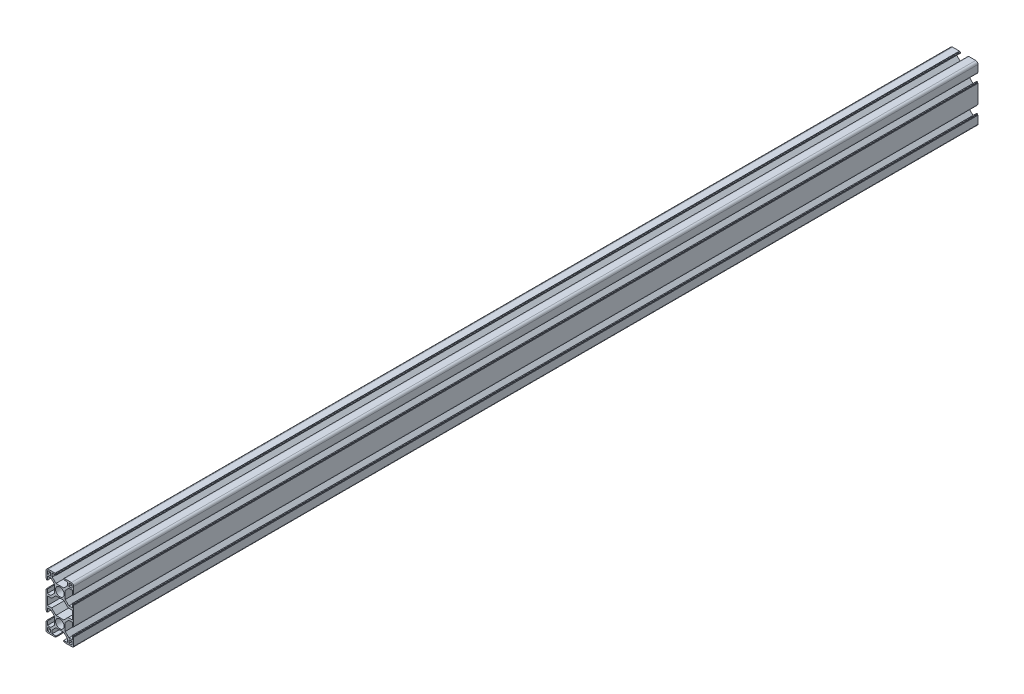
from build123d import *

# Parameters (mm, degrees)
SKETCH1_R                 = 4.6
SKETCH1_W                 = 3.5
SKETCH1_H                 = 3.5
F_30_X_60L_X_R2_5_1_DEPTH = 980


with BuildPart() as part:
    # Sketch1 → 铝型材 30 X 60L X R2.5(1) (new body)
    with BuildSketch(Plane(origin=(0, 0, 0), x_dir=(-1, 0, 0), z_dir=(0, 0, -1))):
        with BuildLine():
            Line((-5.1, 15), (-5.1, 14.5))
            Line((-5.1, 14.5), (-4.1, 14.5))
            Line((-4.1, 14.5), (-4.1, 13.5))
            Line((-4.1, 13.5), (-8.25, 13.5))
            Line((-8.25, 13.5), (-8.25, 9.8))
            Line((-8.25, 9.8), (-4.25, 5.8))
            Line((-4.25, 5.8), (4.25, 5.8))
            Line((4.25, 5.8), (8.25, 9.8))
            Line((8.25, 9.8), (8.25, 13.5))
            Line((8.25, 13.5), (4.1, 13.5))
            Line((4.1, 13.5), (4.1, 14.5))
            Line((4.1, 14.5), (5.1, 14.5))
            Line((5.1, 14.5), (5.1, 15))
            Line((5.1, 15), (12.5, 15))
            ThreePointArc((12.5, 15), (14.267766953, 14.267766953), (15, 12.5))
            Line((15, 12.5), (15, 5.1))
            Line((15, 5.1), (14.5, 5.1))
            Line((14.5, 5.1), (14.5, 4.1))
            Line((14.5, 4.1), (13.5, 4.1))
            Line((13.5, 4.1), (13.5, 8.25))
            Line((13.5, 8.25), (9.8, 8.25))
            Line((9.8, 8.25), (5.8, 4.25))
            Line((5.8, 4.25), (5.8, -4.25))
            Line((5.8, -4.25), (9.8, -8.25))
            Line((9.8, -8.25), (13.5, -8.25))
            Line((13.5, -8.25), (13.5, -4.1))
            Line((13.5, -4.1), (14.5, -4.1))
            Line((14.5, -4.1), (14.5, -5.1))
            Line((14.5, -5.1), (15, -5.1))
            Line((15, -5.1), (15, -24.9))
            Line((15, -24.9), (14.5, -24.9))
            Line((14.5, -24.9), (14.5, -25.9))
            Line((14.5, -25.9), (13.5, -25.9))
            Line((13.5, -25.9), (13.5, -21.75))
            Line((13.5, -21.75), (9.8, -21.75))
            Line((9.8, -21.75), (5.8, -25.75))
            Line((5.8, -25.75), (5.8, -34.25))
            Line((5.8, -34.25), (9.8, -38.25))
            Line((9.8, -38.25), (13.5, -38.25))
            Line((13.5, -38.25), (13.5, -34.1))
            Line((13.5, -34.1), (14.5, -34.1))
            Line((14.5, -34.1), (14.5, -35.1))
            Line((14.5, -35.1), (15, -35.1))
            Line((15, -35.1), (15, -43.5))
            ThreePointArc((15, -43.5), (14.560660172, -44.560660172), (13.5, -45))
            Line((13.5, -45), (5.1, -45))
            Line((5.1, -45), (5.1, -44.5))
            Line((5.1, -44.5), (4.1, -44.5))
            Line((4.1, -44.5), (4.1, -43.5))
            Line((4.1, -43.5), (8.25, -43.5))
            Line((8.25, -43.5), (8.25, -39.8))
            Line((8.25, -39.8), (4.25, -35.8))
            Line((4.25, -35.8), (-4.25, -35.8))
            Line((-4.25, -35.8), (-8.25, -39.8))
            Line((-8.25, -39.8), (-8.25, -43.5))
            Line((-8.25, -43.5), (-4.1, -43.5))
            Line((-4.1, -43.5), (-4.1, -44.5))
            Line((-4.1, -44.5), (-5.1, -44.5))
            Line((-5.1, -44.5), (-5.1, -45))
            Line((-5.1, -45), (-13.5, -45))
            ThreePointArc((-13.5, -45), (-14.560660172, -44.560660172), (-15, -43.5))
            Line((-15, -43.5), (-15, -35.1))
            Line((-15, -35.1), (-14.5, -35.1))
            Line((-14.5, -35.1), (-14.5, -34.1))
            Line((-14.5, -34.1), (-13.5, -34.1))
            Line((-13.5, -34.1), (-13.5, -38.25))
            Line((-13.5, -38.25), (-9.8, -38.25))
            Line((-9.8, -38.25), (-5.8, -34.25))
            Line((-5.8, -34.25), (-5.8, -25.75))
            Line((-5.8, -25.75), (-9.8, -21.75))
            Line((-9.8, -21.75), (-13.5, -21.75))
            Line((-13.5, -21.75), (-13.5, -25.9))
            Line((-13.5, -25.9), (-14.5, -25.9))
            Line((-14.5, -25.9), (-14.5, -24.9))
            Line((-14.5, -24.9), (-15, -24.9))
            Line((-15, -24.9), (-15, -5.1))
            Line((-15, -5.1), (-14.5, -5.1))
            Line((-14.5, -5.1), (-14.5, -4.1))
            Line((-14.5, -4.1), (-13.5, -4.1))
            Line((-13.5, -4.1), (-13.5, -8.25))
            Line((-13.5, -8.25), (-9.8, -8.25))
            Line((-9.8, -8.25), (-5.8, -4.25))
            Line((-5.8, -4.25), (-5.8, 4.25))
            Line((-5.8, 4.25), (-9.8, 8.25))
            Line((-9.8, 8.25), (-13.5, 8.25))
            Line((-13.5, 8.25), (-13.5, 4.1))
            Line((-13.5, 4.1), (-14.5, 4.1))
            Line((-14.5, 4.1), (-14.5, 5.1))
            Line((-14.5, 5.1), (-15, 5.1))
            Line((-15, 5.1), (-15, 12.5))
            ThreePointArc((-15, 12.5), (-14.267766953, 14.267766953), (-12.5, 15))
            Line((-12.5, 15), (-5.1, 15))
        make_face()
        Circle(SKETCH1_R, mode=Mode.SUBTRACT)
        with Locations((0, -30)):
            Circle(SKETCH1_R, mode=Mode.SUBTRACT)
        Polygon((8.9, -10.45), (4.25, -5.8), (-4.25, -5.8), (-8.9, -10.45), (-13.5, -10.45), (-13.5, -19.55), (-8.9, -19.55), (-4.25, -24.2), (4.25, -24.2), (8.9, -19.55), (13.5, -19.55), (13.5, -10.45), align=None, mode=Mode.SUBTRACT)
        with Locations((-11.625, 11.625)):
            Rectangle(SKETCH1_W, SKETCH1_H, mode=Mode.SUBTRACT)
        with Locations((11.625, 11.625)):
            Rectangle(SKETCH1_W, SKETCH1_H, mode=Mode.SUBTRACT)
        with Locations((-11.625, -41.625)):
            Rectangle(SKETCH1_W, SKETCH1_H, mode=Mode.SUBTRACT)
        with Locations((11.625, -41.625)):
            Rectangle(SKETCH1_W, SKETCH1_H, mode=Mode.SUBTRACT)
    extrude(amount=F_30_X_60L_X_R2_5_1_DEPTH)


solid = part.part
